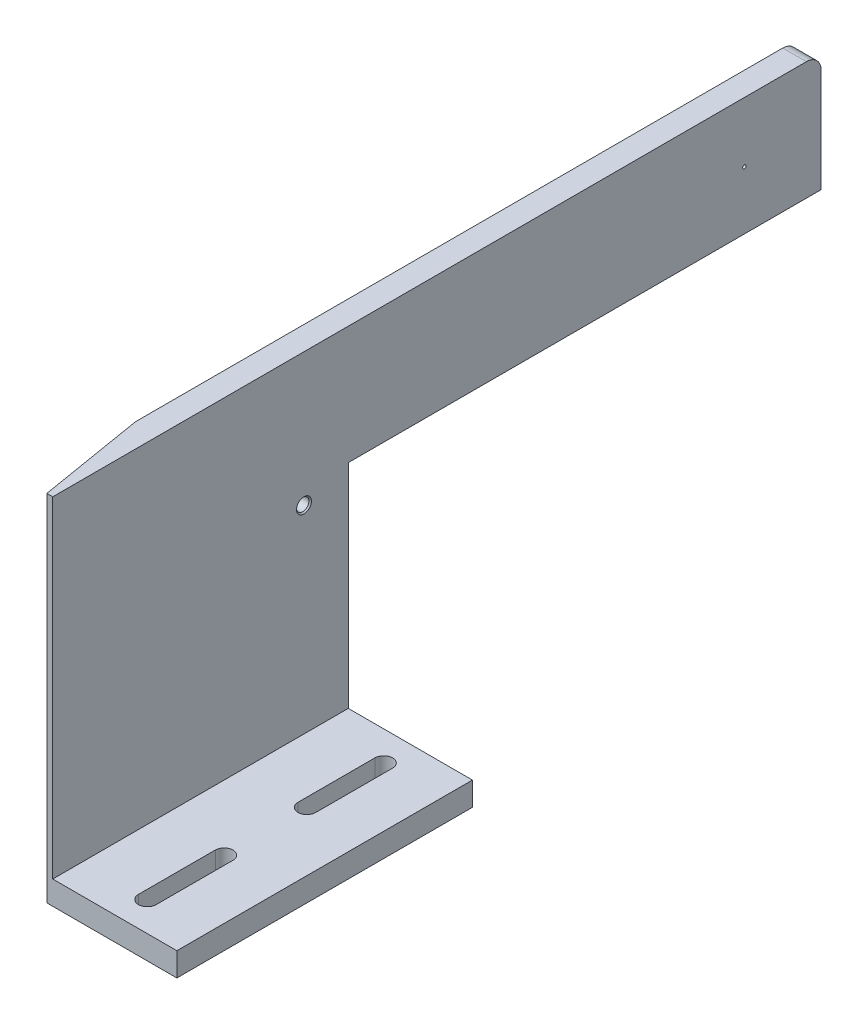
SolidWorks part; units mm, degrees
ref_plane "Front Plane" through (0, 0, 0) normal (0, 0, 1) x (1, 0, 0)
ref_plane "Top Plane" through (0, 0, 0) normal (0, 1, 0) x (1, 0, 0)
ref_plane "Right Plane" through (0, 0, 0) normal (1, 0, 0) x (0, 0, -1)
sketch "Sketch1" plane through (0, 0, 0) normal (0, 0, 1) x (1, 0, 0)
  line L0 (0, 0) -> (0, 120)
  line L1 (0, 0) -> (50, 0)
  line L2 (8, 8) -> (50, 8)
  line L3 (8, 8) -> (8, 120)
  line L4 (50, 8) -> (50, 0)
  line L5 (8, 120) -> (0, 120)
  dimension "D1" = 120
  dimension "D2" = 50
  dimension "D3" = 8
extrude "Boss-Extrude1" add sketch "Sketch1" along normal blind 260
sketch "Sketch2" plane through (50, 0, 0) normal (1, 0, 0) x (0, 0, -1)
  line L0 (-260, 0) -> (0, 0) construction
  line L1 (0, 0) -> (-160, 0)
  line L2 (0, 0) -> (0, 80)
  line L3 (0, 80) -> (-160, 80)
  line L4 (-160, 0) -> (-160, 80)
  dimension "D1" = 80
  dimension "D2" = 160
extrude "Cut-Extrude1" cut sketch "Sketch2" against normal through all
sketch "Sketch3" plane through (0, 8, 0) normal (0, 1, 0) x (1, 0, 0)
  line L0 (30, -250) -> (30, -224) construction
  line L1 (27, -250) -> (27, -224)
  line L2 (33, -250) -> (33, -224)
  line L3 (30, -196) -> (30, -170) construction
  line L4 (27, -196) -> (27, -170)
  line L5 (33, -196) -> (33, -170)
  line L6 (50, -260) -> (50, -160) construction
  line L8 (50, 0) -> (8, 0) construction
  line L9 (50, -260) -> (8, -260) construction
  arc A0 (27, -250) -> (33, -250) centre (30, -250) ccw
  arc A1 (33, -224) -> (27, -224) centre (30, -224) ccw
  arc A2 (27, -196) -> (33, -196) centre (30, -196) ccw
  arc A3 (33, -170) -> (27, -170) centre (30, -170) ccw
  point P2 (30, -237)
  point P7 (30, -183)
  dimension "D4" = 26
  dimension "D5" = 26
  dimension "D6" = 10
  dimension "D7" = 170
  dimension "D1" = 6
  dimension "D2" = 6
  dimension "D3" = 20
extrude "Cut-Extrude2" cut sketch "Sketch3" against normal blind 220
sketch "Sketch4" plane through (0, 120, 0) normal (0, 1, 0) x (1, 0, 0)
  line L0 (6, -260) -> (0, -224)
  line L1 (8, -260) -> (0, -260) construction
  line L2 (0, -260) -> (0, 0) construction
  line L3 (0, -224) -> (0, -260)
  line L4 (0, -260) -> (6, -260)
  dimension "D1" = 6
  dimension "D2" = 36
extrude "Cut-Extrude3" cut sketch "Sketch4" against normal through all
hole_wizard "M5 Tapped Hole1" positions "3DSketch1" profile "Sketch5" tap size "M5" standard "GB"
sketch3d "3DSketch1"
  line L0 (8, 80, 160) -> (8, 80, 0) construction
  line L1 (8, 8, 160) -> (8, 80, 160) construction
  point P0 (8, 75, 175)
  dimension "D1" = 5
  dimension "D2" = 15
sketch "Sketch5" plane through (8, 75, 175) normal (0, 1, 0) x (0, 0, -1)
  line L0 (0, 0) -> (0, 7.2618)
  line L1 (0, 7.2618) -> (2.1, 6)
  line L2 (2.1, 6) -> (2.1, 0.425)
  line L3 (2.1, 0.425) -> (2.525, 0)
  line L5 (2.525, 0) -> (0, 0)
  line L6 (-2.1, 0.425) -> (-2.525, 0) construction
  line L10 (0, 7.2618) -> (-2.1, 6) construction
  line L11 (0, -6.35) -> (0, 107.95) construction
  dimension "螺纹孔钻头直径" = 4.2
  dimension "螺纹孔钻头深度" = 6
  dimension "近端锥形沉头孔直径" = 5.05
  dimension "近端锥形沉头孔角度" = 90
  dimension "导头角度" = 118
cosmetic thread "Hole Thread Line1" parameters "D1"=5, "D2"=5
fillet "Fillet1" radius 5 1 edges at (4, 120, 0)
sketch "Sketch6" plane through (8, 0, 0) normal (1, 0, 0) x (0, 0, -1)
  line L1 (-26, 119.36) -> (-26, 80) construction
  line L2 (-160, 80) -> (0, 80) construction
  line L3 (0, 80) -> (0, 115) construction
  circle A0 centre (-26, 99.68) radius 0.6
  dimension "D1" = 1.2
  dimension "D2" = 26
extrude "Cut-Extrude4" cut sketch "Sketch6" against normal through all
